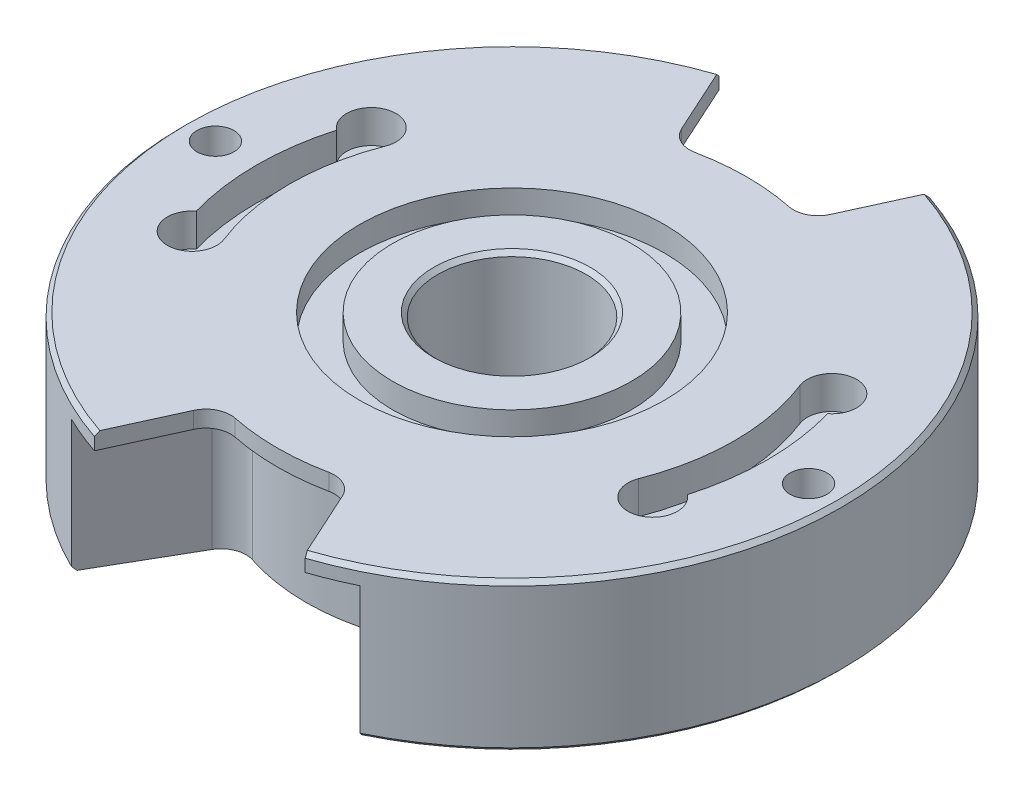
from build123d import *

# Parameters (mm, degrees)
SKETCH1_R               = 40
BOSS_EXTRUDE1_DEPTH     = 18
CHAMFER2_SIZE           = 0.5
CUT_EXTRUDE1_DEPTH      = 60.363288319
CUT_EXTRUDE1_DEPTH_BACK = 60.363288319
SKETCH2_R               = 2.25
CUT_EXTRUDE2_DEPTH      = 4
CUT_EXTRUDE3_DEPTH      = 60.363288319
SKETCH5_R               = 9
CUT_EXTRUDE4_DEPTH      = 58.967380496
CUT_EXTRUDE5_DEPTH      = 16
SKETCH7_R               = 18.5
SKETCH7_R_2             = 14.5
CUT_EXTRUDE6_DEPTH      = 3
CHAMFER1_SIZE           = 0.5


with BuildPart() as part:
    # Sketch1 → Boss-Extrude1 (new body)
    with BuildSketch(Plane(origin=(0, 0, 0), x_dir=(1, 0, 0), z_dir=(0, 1, 0))):
        with Locations(Location((0, 0, 0), (0, 0, 270))):
            Circle(SKETCH1_R)
    extrude(amount=BOSS_EXTRUDE1_DEPTH)

    # Chamfer2
    chamfer2_edges = [part.edges().sort_by_distance(p)[0] for p in [
        (0, 0, -40),
        (0, 18, -40),
    ]]
    chamfer(chamfer2_edges, length=CHAMFER2_SIZE)

    # Sketch2 → Cut-Extrude1 (cut, two sides: drawn at the far end of the back side and taken through both)
    with BuildSketch(Plane(origin=(0, 18, 0), x_dir=(1, 0, 0), z_dir=(0, 1, 0)).offset(-CUT_EXTRUDE1_DEPTH_BACK)):
        with Locations(Location((36, 0, 0), (0, 0, 270))):
            Circle(SKETCH2_R)
        with Locations(Location((-36, 0, 0), (0, 0, 270))):
            Circle(SKETCH2_R)
    extrude(amount=CUT_EXTRUDE1_DEPTH + CUT_EXTRUDE1_DEPTH_BACK, mode=Mode.SUBTRACT)

    # Sketch3 → Cut-Extrude2 (cut)
    with BuildSketch(Plane(origin=(0, 18, 0), x_dir=(1, 0, 0), z_dir=(0, 1, 0))):
        with BuildLine():
            ThreePointArc((-25.162362394, 9.790583167), (-27, 0), (-25.162362394, -9.790583167))
            ThreePointArc((-25.162362394, -9.790583167), (-28.751993608, -13.771496887), (-29.807321036, -8.516079652))
            ThreePointArc((-29.807321036, -8.516079652), (-31, 0), (-29.807321036, 8.516079652))
            ThreePointArc((-29.807321036, 8.516079652), (-28.751993608, 13.771496887), (-25.162362394, 9.790583167))
        make_face()
        with BuildLine():
            ThreePointArc((25.162362394, -9.790583167), (28.751993608, -13.771496887), (29.807321036, -8.516079652))
            ThreePointArc((29.807321036, -8.516079652), (31, 0), (29.807321036, 8.516079652))
            ThreePointArc((29.807321036, 8.516079652), (28.751993608, 13.771496887), (25.162362394, 9.790583167))
            ThreePointArc((25.162362394, 9.790583167), (27, 0), (25.162362394, -9.790583167))
        make_face()
    extrude(amount=-CUT_EXTRUDE2_DEPTH, mode=Mode.SUBTRACT)

    # Sketch4 → Cut-Extrude3 (cut, through all)
    with BuildSketch(Plane(origin=(0, 18, 0), x_dir=(1, 0, 0), z_dir=(0, 1, 0))):
        with BuildLine():
            Line((-12.797765369, 37.8974564), (-9.02567097, 29.620350674))
            ThreePointArc((-9.02567097, 29.620350674), (-7.657078917, 28.191064594), (-5.696188381, 27.92496084))
            ThreePointArc((-5.696188381, 27.92496084), (0, 28.5), (5.696188381, 27.92496084))
            ThreePointArc((5.696188381, 27.92496084), (7.657078917, 28.191064594), (9.02567097, 29.620350674))
            Line((9.02567097, 29.620350674), (12.797765369, 37.8974564))
            ThreePointArc((12.797765369, 37.8974564), (0, 40), (-12.797765369, 37.8974564))
        make_face()
        with BuildLine():
            Line((12.797765369, -37.8974564), (9.02567097, -29.620350674))
            ThreePointArc((9.02567097, -29.620350674), (7.657078917, -28.191064594), (5.696188381, -27.92496084))
            ThreePointArc((5.696188381, -27.92496084), (0, -28.5), (-5.696188381, -27.92496084))
            ThreePointArc((-5.696188381, -27.92496084), (-7.657078917, -28.191064594), (-9.02567097, -29.620350674))
            Line((-9.02567097, -29.620350674), (-12.797765369, -37.8974564))
            ThreePointArc((-12.797765369, -37.8974564), (0, -40), (12.797765369, -37.8974564))
        make_face()
    extrude(amount=-CUT_EXTRUDE3_DEPTH, mode=Mode.SUBTRACT)

    # Sketch5 → Cut-Extrude4 (cut, through all)
    with BuildSketch(Plane(origin=(0, 0, 0), x_dir=(-1, 0, 0), z_dir=(0, -1, 0))):
        with Locations(Location((0, 0, 0), (0, 0, 90))):
            Circle(SKETCH5_R)
    extrude(amount=-CUT_EXTRUDE4_DEPTH, mode=Mode.SUBTRACT)

    # Sketch6 → Cut-Extrude5 (cut)
    with BuildSketch(Plane(origin=(0, 0, 0), x_dir=(-1, 0, 0), z_dir=(0, -1, 0))):
        with BuildLine():
            Line((17.529506166, -35.95436571), (11.275186187, -25.12156574))
            ThreePointArc((11.275186187, -25.12156574), (9.750918079, -23.820327414), (7.747419621, -23.769255125))
            ThreePointArc((7.747419621, -23.769255125), (0, -25), (-7.747419621, -23.769255125))
            ThreePointArc((-7.747419621, -23.769255125), (-9.750918079, -23.820327414), (-11.275186187, -25.12156574))
            Line((-11.275186187, -25.12156574), (-17.529506166, -35.95436571))
            ThreePointArc((-17.529506166, -35.95436571), (0, -40), (17.529506166, -35.95436571))
        make_face()
        with BuildLine():
            Line((-17.529506166, 35.95436571), (-11.275186187, 25.12156574))
            ThreePointArc((-11.275186187, 25.12156574), (-9.750918079, 23.820327414), (-7.747419621, 23.769255125))
            ThreePointArc((-7.747419621, 23.769255125), (0, 25), (7.747419621, 23.769255125))
            ThreePointArc((7.747419621, 23.769255125), (9.750918079, 23.820327414), (11.275186187, 25.12156574))
            Line((11.275186187, 25.12156574), (17.529506166, 35.95436571))
            ThreePointArc((17.529506166, 35.95436571), (0, 40), (-17.529506166, 35.95436571))
        make_face()
    extrude(amount=-CUT_EXTRUDE5_DEPTH, mode=Mode.SUBTRACT)

    # Sketch7 → Cut-Extrude6 (cut)
    with BuildSketch(Plane(origin=(0, 18, 0), x_dir=(1, 0, 0), z_dir=(0, 1, 0))):
        with Locations(Location((0, 0, 0), (0, 0, 270))):
            Circle(SKETCH7_R)
        with Locations(Location((0, 0, 0), (0, 0, 270))):
            Circle(SKETCH7_R_2, mode=Mode.SUBTRACT)
    extrude(amount=-CUT_EXTRUDE6_DEPTH, mode=Mode.SUBTRACT)

    # Chamfer1
    chamfer1_edges = [part.edges().sort_by_distance(p)[0] for p in [
        (0, 18, 9),
        (0, 0, 9),
    ]]
    chamfer(chamfer1_edges, length=CHAMFER1_SIZE)


solid = part.part
